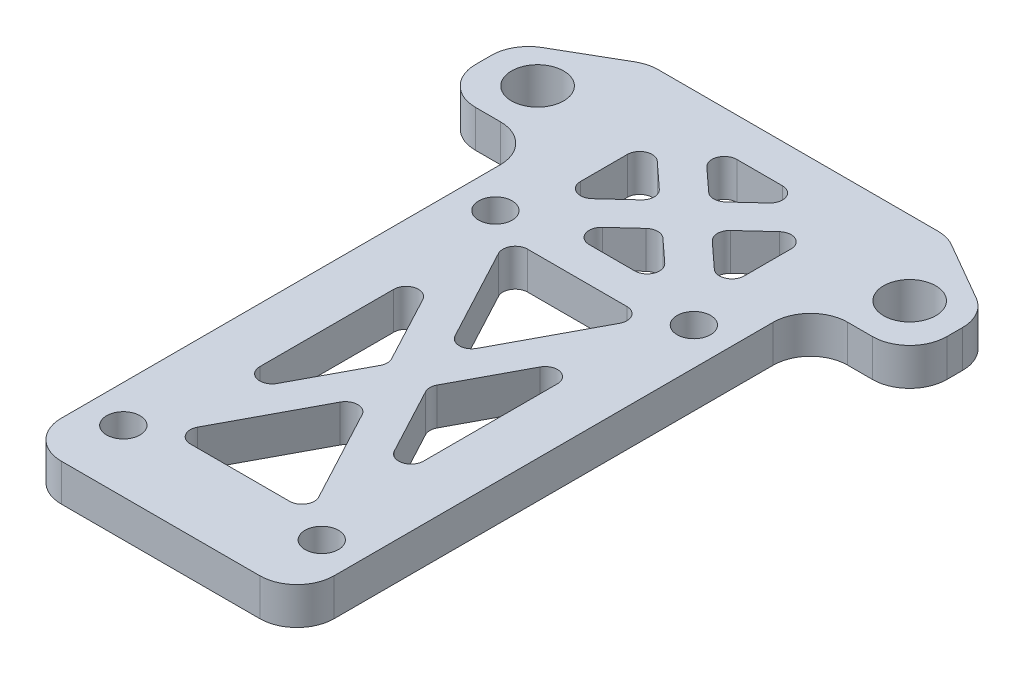
SolidWorks part; units mm, degrees
material "Thornel Mat VMA"
ref_plane "Front Plane" through (0, 0, 0) normal (0, 0, 1) x (1, 0, 0)
ref_plane "Top Plane" through (0, 0, 0) normal (0, 1, 0) x (1, 0, 0)
ref_plane "Right Plane" through (0, 0, 0) normal (1, 0, 0) x (0, 0, -1)
sketch "Sketch1" plane through (0, 0, 0) normal (0, 1, 0) x (1, 0, 0)
  line L0 (0, 6) -> (0, -45.4) construction
  line L2 (-12.0718, 6) -> (-19, 2)
  line L3 (-19, 2) -> (-19, -4)
  line L4 (-19, -4) -> (-11, -4)
  line L5 (-11, -4) -> (-11, -45.4)
  line L6 (-11, -45.4) -> (11, -45.4)
  line L7 (12.0718, 6) -> (19, 2)
  line L8 (19, 2) -> (19, -4)
  line L9 (19, -4) -> (11, -4)
  line L10 (11, -4) -> (11, -45.4)
  line L19 (12.0718, 6) -> (-12.0718, 6)
  circle A0 centre (-15, 0) radius 2.1
  circle A1 centre (15, 0) radius 2.1
  circle A2 centre (-8, -10.4) radius 1.35
  circle A3 centre (-8, -40.4) radius 1.35
  circle A4 centre (8, -10.4) radius 1.35
  circle A5 centre (8, -40.4) radius 1.35
  dimension "D2" = 4.2
  dimension "D3" = 2.7
  dimension "D4" = 30
  dimension "D5" = 30
  dimension "D6" = 16
  dimension "D7" = 6.4
  dimension "D8" = 4
  dimension "D9" = 38
  dimension "D10" = 22
  dimension "D11" = 5
  dimension "D12" = 6
  dimension "D13" = 120
  dimension "D14" = 6
extrude "Boss-Extrude1" add sketch "Sketch1" along normal blind 3
sketch "Sketch2" plane through (0, 3, 0) normal (0, 1, 0) x (1, 0, 0)
  line L0 (-8, -10.4) -> (8, -40.4) construction
  line L1 (-6.7647, -9.7412) -> (9.2353, -39.7412)
  line L2 (-9.2353, -11.0588) -> (6.7647, -41.0588)
  line L3 (8, -10.4) -> (-8, -40.4) construction
  line L4 (9.2353, -11.0588) -> (-6.7647, -41.0588)
  line L5 (6.7647, -9.7412) -> (-9.2353, -39.7412)
  line L6 (-8, -10.4) -> (8, -10.4) construction
  line L7 (-8, -9) -> (8, -9)
  line L8 (-8, -11.8) -> (8, -11.8)
  line L9 (8, -10.4) -> (8, -40.4) construction
  line L10 (9.4, -10.4) -> (9.4, -40.4)
  line L11 (6.6, -10.4) -> (6.6, -40.4)
  line L12 (8, -40.4) -> (-8, -40.4) construction
  line L13 (8, -41.8) -> (-8, -41.8)
  line L14 (8, -39) -> (-8, -39)
  line L15 (-8, -40.4) -> (-8, -10.4) construction
  line L16 (-9.4, -40.4) -> (-9.4, -10.4)
  line L17 (-6.6, -40.4) -> (-6.6, -10.4)
  line L18 (-8, 4.3) -> (8, 4.3) construction
  line L19 (-8, 5.7) -> (8, 5.7)
  line L20 (-8, 2.9) -> (8, 2.9)
  line L21 (-8, 4.3) -> (-8, -10.4) construction
  line L22 (-6.6, 4.3) -> (-6.6, -10.4)
  line L23 (-9.4, 4.3) -> (-9.4, -10.4)
  line L24 (8, -10.4) -> (8, 4.3) construction
  line L25 (6.6, -10.4) -> (6.6, 4.3)
  line L26 (9.4, -10.4) -> (9.4, 4.3)
  line L27 (-8, 4.3) -> (8, -10.4) construction
  line L28 (-7.0528, 5.3309) -> (8.9472, -9.3691)
  line L29 (-8.9472, 3.2691) -> (7.0528, -11.4309)
  line L30 (8, 4.3) -> (-8, -10.4) construction
  line L31 (8.9472, 3.2691) -> (-7.0528, -11.4309)
  line L32 (7.0528, 5.3309) -> (-8.9472, -9.3691)
  line L34 (12.0718, 6) -> (-12.0718, 6) construction
  arc A0 (-6.7647, -9.7412) -> (-9.2353, -11.0588) centre (-8, -10.4) ccw
  arc A1 (6.7647, -41.0588) -> (9.2353, -39.7412) centre (8, -40.4) ccw
  arc A2 (9.2353, -11.0588) -> (6.7647, -9.7412) centre (8, -10.4) ccw
  arc A3 (-9.2353, -39.7412) -> (-6.7647, -41.0588) centre (-8, -40.4) ccw
  arc A4 (-8, -9) -> (-8, -11.8) centre (-8, -10.4) ccw
  arc A5 (8, -11.8) -> (8, -9) centre (8, -10.4) ccw
  arc A6 (9.4, -10.4) -> (6.6, -10.4) centre (8, -10.4) ccw
  arc A7 (6.6, -40.4) -> (9.4, -40.4) centre (8, -40.4) ccw
  arc A8 (8, -41.8) -> (8, -39) centre (8, -40.4) ccw
  arc A9 (-8, -39) -> (-8, -41.8) centre (-8, -40.4) ccw
  arc A10 (-9.4, -40.4) -> (-6.6, -40.4) centre (-8, -40.4) ccw
  arc A11 (-6.6, -10.4) -> (-9.4, -10.4) centre (-8, -10.4) ccw
  arc A12 (-8, 5.7) -> (-8, 2.9) centre (-8, 4.3) ccw
  arc A13 (8, 2.9) -> (8, 5.7) centre (8, 4.3) ccw
  arc A14 (-6.6, 4.3) -> (-9.4, 4.3) centre (-8, 4.3) ccw
  arc A15 (-9.4, -10.4) -> (-6.6, -10.4) centre (-8, -10.4) ccw
  arc A16 (6.6, -10.4) -> (9.4, -10.4) centre (8, -10.4) ccw
  arc A17 (9.4, 4.3) -> (6.6, 4.3) centre (8, 4.3) ccw
  arc A18 (-7.0528, 5.3309) -> (-8.9472, 3.2691) centre (-8, 4.3) ccw
  arc A19 (7.0528, -11.4309) -> (8.9472, -9.3691) centre (8, -10.4) ccw
  arc A20 (8.9472, 3.2691) -> (7.0528, 5.3309) centre (8, 4.3) ccw
  arc A21 (-8.9472, -9.3691) -> (-7.0528, -11.4309) centre (-8, -10.4) ccw
  point P4 (0, -25.4)
  point P9 (0, -25.4)
  point P20 (0, -10.4)
  point P25 (8, -25.4)
  point P32 (0, -40.4)
  point P39 (-8, -25.4)
  point P48 (0, 4.3)
  point P53 (-8, -3.05)
  point P60 (8, -3.05)
  point P67 (0, -3.05)
  point P74 (0, -3.05)
  dimension "D1" = 1.4
  dimension "D2" = 0.3
extrude "Cut-Extrude1" cut sketch "Sketch2" against normal through all contours L32 L29 L22 | L32 L20 L28 | L25 L31 L28 | L29 L31 L7 | L8 L1 L5 | L17 L5 L2 | L14 L2 L4 | L11 L4 L1
fillet "R3 outer edge fillet" radius 3 10 edges at (11, 1.5, 45.4) (11, 1.5, 4) (19, 1.5, 4) (19, 1.5, -2) (-19, 1.5, -2) (-19, 1.5, 4) (-11, 1.5, 4) (-11, 1.5, 45.4) (-12.0718, 1.5, -6) (12.0718, 1.5, -6)
fillet "R1 cutout fillet" radius 1 24 edges at (6.6, 1.5, 34.8) (6.6, 1.5, 16) (1.5867, 1.5, 25.4) (5.6667, 1.5, 39) (0, 1.5, 28.375) (-5.6667, 1.5, 39) (-6.6, 1.5, 34.8) (-1.5867, 1.5, 25.4) (-6.6, 1.5, 16) (0, 1.5, 22.425) (5.6667, 1.5, 11.8) (-5.6667, 1.5, 11.8) (4.4069, 1.5, -2.9) (0, 1.5, 1.1488) (-4.4069, 1.5, -2.9) (2.0693, 1.5, 3.05) (6.6, 1.5, -1.1126) (6.6, 1.5, 7.2126) (4.4069, 1.5, 9) (0, 1.5, 4.9512) (-4.4069, 1.5, 9) (-6.6, 1.5, 7.2126) (-2.0693, 1.5, 3.05) (-6.6, 1.5, -1.1126)
